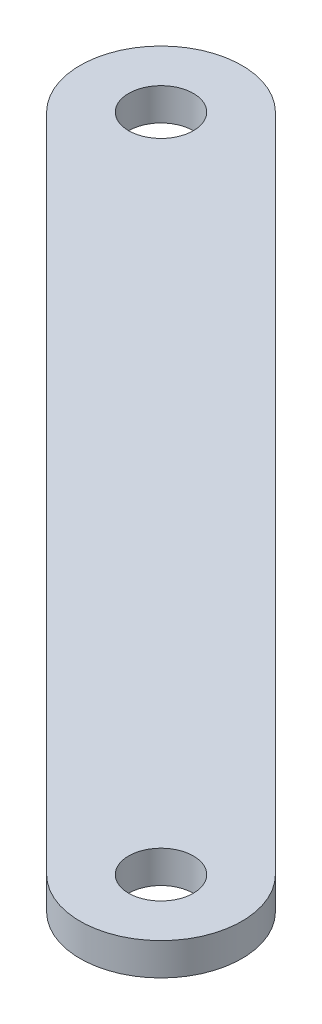
from build123d import *

# Parameters (mm, degrees)
SKETCH1_R          = 4
BOSS_EXTRU_1_DEPTH = 4


with BuildPart() as part:
    # Sketch1 → Boss.-Extru.1 (new body)
    with BuildSketch(Plane(origin=(0, 0, 0), x_dir=(1, 0, 0), z_dir=(0, 1, 0))):
        with BuildLine():
            Line((38.094109607, -47.888548123), (-43.540851016, 33.7464125))
            ThreePointArc((-43.540851016, 33.7464125), (-43.540851016, 47.888548123), (-29.398715392, 47.888548123))
            Line((-29.398715392, 47.888548123), (52.236245231, -33.7464125))
            ThreePointArc((52.236245231, -33.7464125), (52.236245231, -47.888548123), (38.094109607, -47.888548123))
        make_face()
        with Locations(Location((45.165177419, -40.817480312, 0), (0, 0, 270))):
            Circle(SKETCH1_R, mode=Mode.SUBTRACT)
        with Locations(Location((-36.469783204, 40.817480312, 0), (0, 0, 270))):
            Circle(SKETCH1_R, mode=Mode.SUBTRACT)
    extrude(amount=BOSS_EXTRU_1_DEPTH)


solid = part.part
